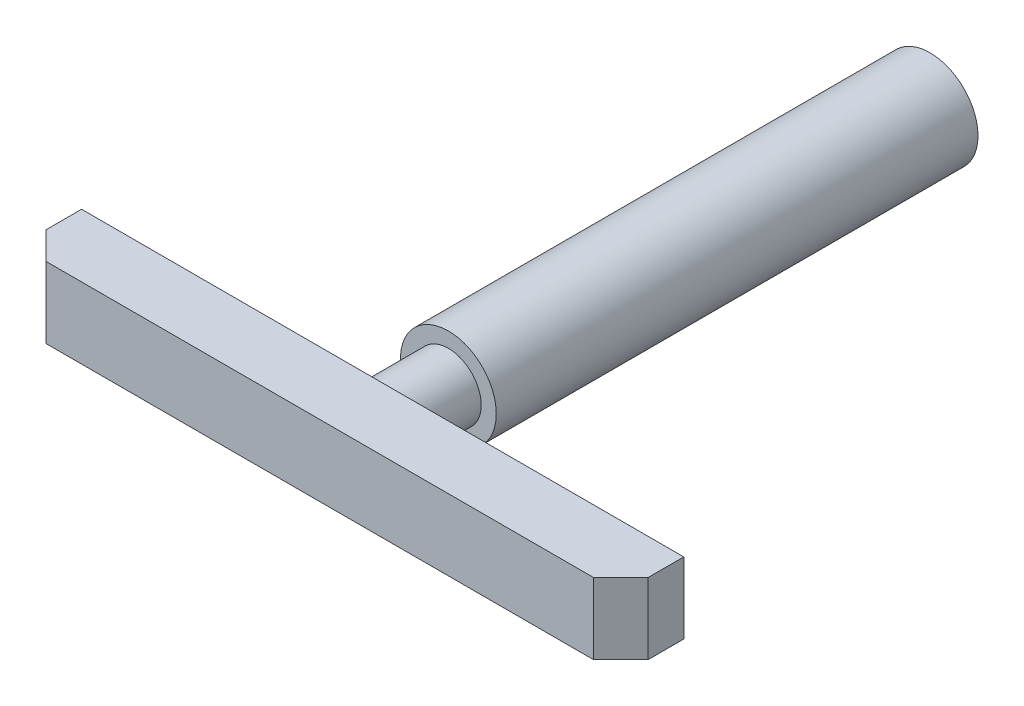
from build123d import *

# Parameters (mm, degrees)
SKETCH1_R           = 17.5
BOSS_EXTRUDE1_DEPTH = 200
SKETCH3_OUTSIDE_W   = 78.206
SKETCH3_OUTSIDE_H   = 78.206
SKETCH3_OUTSIDE_R   = 12
CUT_EXTRUDE1_DEPTH  = 24
SKETCH4_W           = 220
SKETCH4_H           = 26
BOSS_EXTRUDE2_DEPTH = 23
CHAMFER1_SIZE       = 10


with BuildPart() as part:
    # Sketch1 → Boss-Extrude1 (new body)
    with BuildSketch(Plane.XY):
        Circle(SKETCH1_R)
    extrude(amount=BOSS_EXTRUDE1_DEPTH)

    # Sketch3 outside → Cut-Extrude1 (cut)
    with BuildSketch(Plane.XY.offset(200)):
        Rectangle(SKETCH3_OUTSIDE_W, SKETCH3_OUTSIDE_H)
        Circle(SKETCH3_OUTSIDE_R, mode=Mode.SUBTRACT)
    extrude(amount=-CUT_EXTRUDE1_DEPTH, mode=Mode.SUBTRACT)

    # Sketch4 → Boss-Extrude2 (add)
    with BuildSketch(Plane.XY.offset(200)):
        Rectangle(SKETCH4_W, SKETCH4_H)
    extrude(amount=BOSS_EXTRUDE2_DEPTH)

    # Chamfer1
    chamfer1_edges = [part.edges().sort_by_distance(p)[0] for p in [
        (-110, 0, 223),
        (110, 0, 223),
    ]]
    chamfer(chamfer1_edges, length=CHAMFER1_SIZE)


solid = part.part
